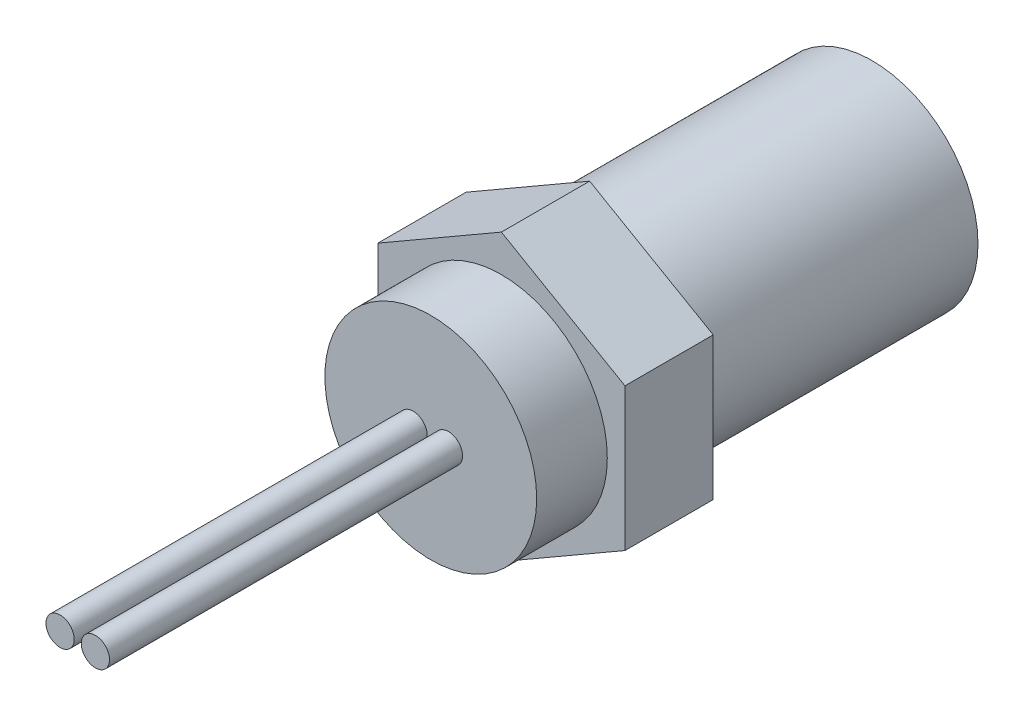
from build123d import *

# Parameters (mm, degrees)
SKETCH1_R           = 3
BOSS_EXTRUDE1_DEPTH = 8
BOSS_EXTRUDE2_DEPTH = 2.5
SKETCH3_R           = 3
BOSS_EXTRUDE3_DEPTH = 2
SKETCH4_R           = 0.4
BOSS_EXTRUDE4_DEPTH = 10


with BuildPart() as part:
    # Sketch1 → Boss-Extrude1 (new body)
    with BuildSketch(Plane.XY):
        Circle(SKETCH1_R)
    extrude(amount=BOSS_EXTRUDE1_DEPTH)

    # Sketch2 → Boss-Extrude2 (add)
    with BuildSketch(Plane.XY.offset(8)):
        Polygon((0, 4.041451884), (-3.5, 2.020725942), (-3.5, -2.020725942), (0, -4.041451884), (3.5, -2.020725942), (3.5, 2.020725942), align=None)
    extrude(amount=BOSS_EXTRUDE2_DEPTH)

    # Sketch3 → Boss-Extrude3 (add)
    with BuildSketch(Plane.XY.offset(10.5)):
        Circle(SKETCH3_R)
    extrude(amount=BOSS_EXTRUDE3_DEPTH)

    # Sketch4 → Boss-Extrude4 (add)
    with BuildSketch(Plane.XY.offset(12.5)):
        with Locations((0.5, 0)):
            Circle(SKETCH4_R)
        with Locations((-0.5, 0)):
            Circle(SKETCH4_R)
    extrude(amount=BOSS_EXTRUDE4_DEPTH)


solid = part.part
